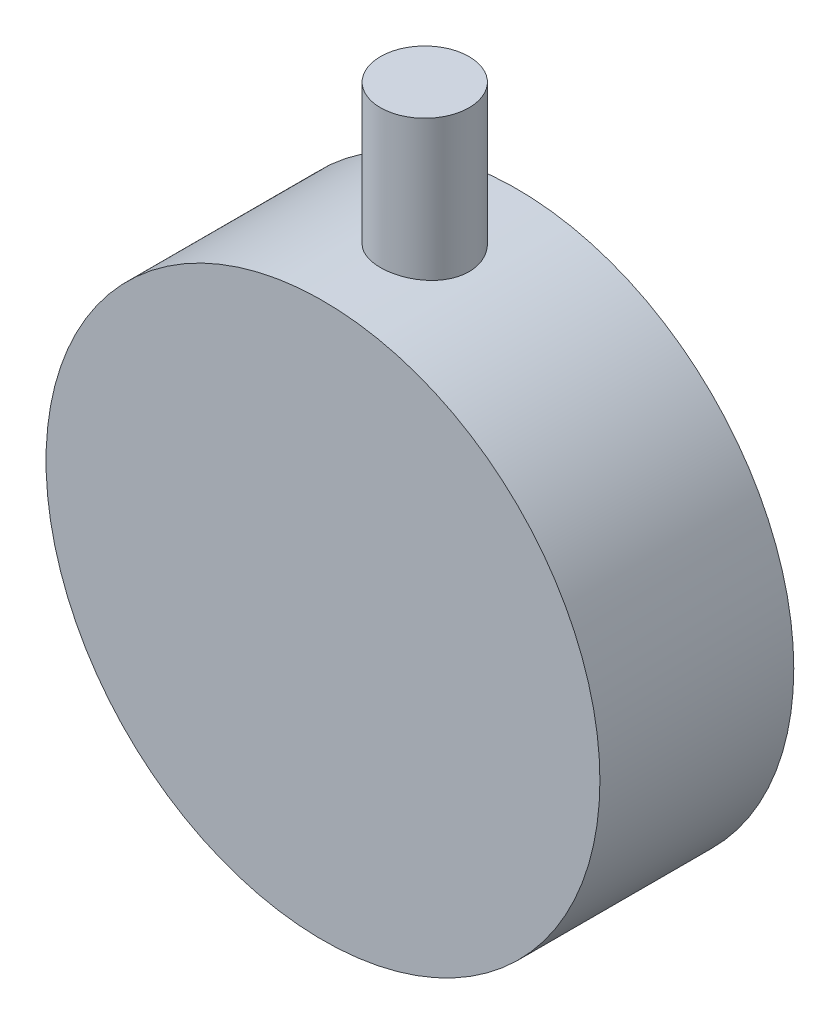
SolidWorks part; units mm, degrees
ref_plane "Front Plane" through (0, 0, 0) normal (0, 0, 1) x (1, 0, 0)
ref_plane "Top Plane" through (0, 0, 0) normal (0, 1, 0) x (1, 0, 0)
ref_plane "Right Plane" through (0, 0, 0) normal (1, 0, 0) x (0, 0, -1)
sketch "Sketch1" plane through (0, 0, 0) normal (0, 0, 1) x (1, 0, 0)
  circle A0 centre (0, 0) radius 50
  dimension "D1" = 100
extrude "Boss-Extrude1" add sketch "Sketch1" along normal blind 35
sketch "Sketch2" plane through (0, 0, 0) normal (0, 1, 0) x (1, 0, 0)
  circle A0 centre (0, -16.6244) radius 8
  dimension "D1" = 16
extrude "Boss-Extrude2" add sketch "Sketch2" along normal blind 75
